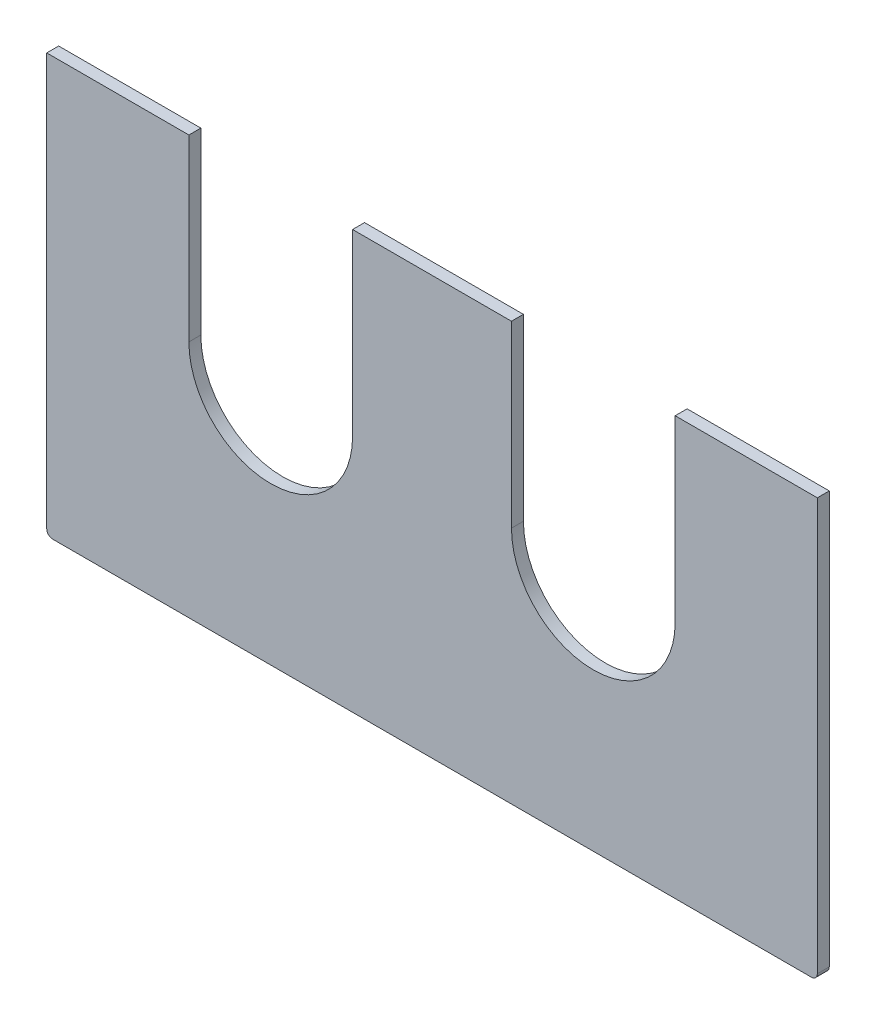
SolidWorks part; units mm, degrees
material "06Cr19Ni10"
ref_plane "Front Plane" through (0, 0, 0) normal (0, 0, 1) x (1, 0, 0)
ref_plane "Top Plane" through (0, 0, 0) normal (0, 1, 0) x (1, 0, 0)
ref_plane "Right Plane" through (0, 0, 0) normal (1, 0, 0) x (0, 0, -1)
sketch "Sketch1" plane through (0, 0, 0) normal (0, 0, 1) x (1, 0, 0)
  line L1 (645, -350) -> (-645, -350)
  line L2 (645, -350) -> (645, 350)
  line L3 (645, 350) -> (-645, 350)
  line L4 (-645, -350) -> (-645, 350)
  line L5 (0, 350) -> (0, -350) construction
  line L6 (645, 0) -> (-645, 0) construction
  point P0 (0, 0)
  dimension "D1" = 1290
  dimension "D2" = 700
extrude "Boss-Extrude1" add sketch "Sketch1" along normal blind 20
sketch "Sketch2" plane through (0, 0, 20) normal (0, 0, 1) x (1, 0, 0)
  line L0 (0, 0) -> (0, 396.1752) construction
  line L1 (645, 350) -> (-645, 350) construction
  line L2 (-407, 50) -> (-407, 350)
  line L3 (-133, 50) -> (-133, 350)
  line L4 (-407, 350) -> (-133, 350)
  line L5 (407, 350) -> (133, 350)
  line L6 (133, 50) -> (133, 350)
  line L7 (407, 50) -> (407, 350)
  arc A0 (-407, 50) -> (-133, 50) centre (-270, 50) ccw
  arc A1 (407, 50) -> (133, 50) centre (270, 50) cw
  dimension "D1" = 540
  dimension "D2" = 274
  dimension "D3" = 300
extrude "Cut-Extrude1" cut sketch "Sketch2" against normal blind 20
fillet "Fillet1" radius 10 2 edges at (645, -350, 10) (-645, -350, 10)
